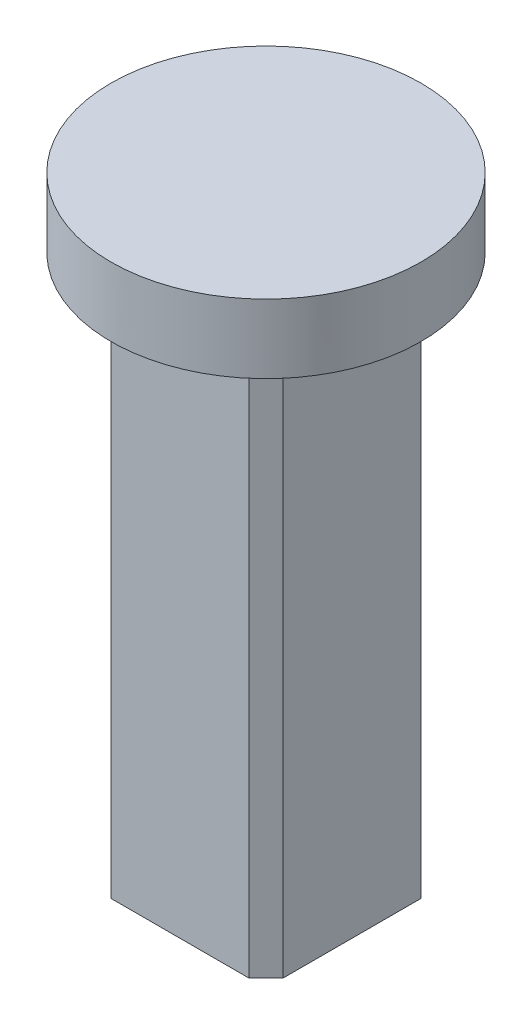
SolidWorks part; units mm, degrees
material "SKD11"
ref_plane "前视" through (0, 0, 0) normal (0, 0, 1) x (1, 0, 0)
ref_plane "上视" through (0, 0, 0) normal (0, 1, 0) x (1, 0, 0)
ref_plane "右视" through (0, 0, 0) normal (1, 0, 0) x (0, 0, -1)
sketch "草图1" plane through (0, 0, 0) normal (0, 1, 0) x (1, 0, 0)
  circle A0 centre (0, 0) radius 4.5
  dimension "D1" = 9
extrude "凸台-拉伸1" add sketch "草图1" along normal mid plane 18
sketch "草图2" plane through (0, -9, 0) normal (0, -1, 0) x (1, 0, 0)
  line L1 (-2.5, -2.5) -> (2.5, -2.5)
  line L2 (-2.5, -2.5) -> (-2.5, 2.5)
  line L3 (-2.5, 2.5) -> (2.5, 2.5)
  line L4 (2.5, -2.5) -> (2.5, 2.5)
  line L5 (-2.5, -2.5) -> (2.5, 2.5) construction
  line L6 (-2.5, 2.5) -> (2.5, -2.5) construction
  circle A0 centre (0, 0) radius 4.5
  point P0 (0, 0)
  dimension "D2" = 9
  dimension "D1" = 5
extrude "切除-拉伸1" cut sketch "草图2" against normal blind 16
hole_wizard "M3 螺纹孔1" positions "草图6" profile "草图7" tap size "M3" standard "GB"
sketch "草图6" plane through (0, -9, 0) normal (0, -1, 0) x (-1, 0, 0)
  point P0 (0, 0)
sketch "草图7" plane through (0, -9, 0) normal (1, 0, 0) x (0, 0, -1)
  line L0 (0, 0) -> (0, 9.2511)
  line L1 (0, 9.2511) -> (1.25, 8.5)
  line L2 (1.25, 8.5) -> (1.25, 0)
  line L5 (1.25, 0) -> (0, 0)
  line L10 (0, 9.2511) -> (-1.25, 8.5) construction
  line L11 (0, -6.35) -> (0, 107.95) construction
  dimension "螺纹孔钻头直径" = 2.5
  dimension "螺纹孔钻头深度" = 8.5
  dimension "导头角度" = 118
cosmetic thread "孔螺蚊线1" parameters "D1"=6, "D2"=3
chamfer "倒角1" distance 0.5 angle 45 4 edges at (-2.5, -1, -2.5) (2.5, -1, -2.5) (-2.5, -1, 2.5) (2.5, -1, 2.5)
